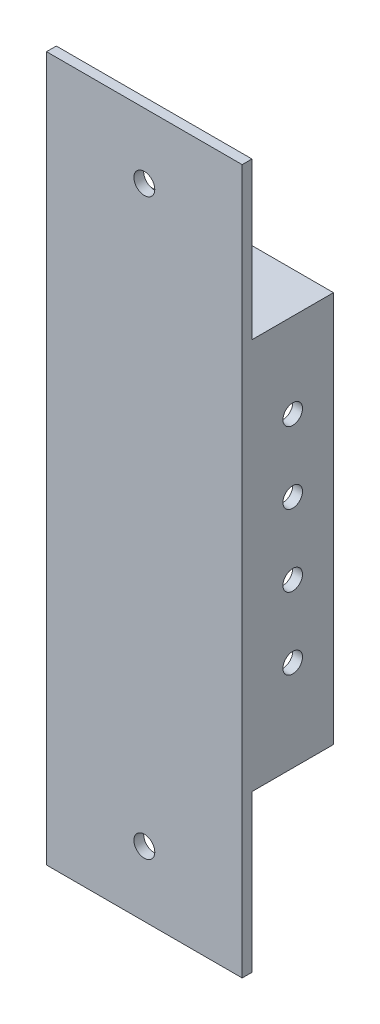
SolidWorks part; units mm, degrees
ref_plane "Front Plane" through (0, 0, 0) normal (0, 0, 1) x (1, 0, 0)
ref_plane "Top Plane" through (0, 0, 0) normal (0, 1, 0) x (1, 0, 0)
ref_plane "Right Plane" through (0, 0, 0) normal (1, 0, 0) x (0, 0, -1)
other "Configuration Table"
sketch "Sketch1" plane through (0, 0, 0) normal (0, 0, 1) x (1, 0, 0)
  line L1 (-300, -600) -> (300, -600)
  line L2 (-300, -600) -> (-300, 600)
  line L3 (-300, 600) -> (300, 600)
  line L4 (300, -600) -> (300, 600)
  line L5 (-300, -600) -> (300, 600) construction
  line L6 (-300, 600) -> (300, -600) construction
  point P0 (0, 0)
  dimension "D1" = 600
  dimension "D2" = 1200
extrude "Boss-Extrude1" add sketch "Sketch1" along normal blind 30
sketch "Sketch3" plane through (0, 0, 0) normal (0, 0, -1) x (-1, 0, 0)
  line L1 (-300, 600) -> (300, 600)
  line L2 (-300, 600) -> (-300, -600)
  line L3 (-300, -600) -> (300, -600)
  line L4 (300, 600) -> (300, -600)
  line L5 (-270, 570) -> (270, 570)
  line L6 (-270, 570) -> (-270, -570)
  line L7 (-270, -570) -> (270, -570)
  line L8 (270, 570) -> (270, -570)
  dimension "D1" = 30
  dimension "D2" = 30
  dimension "D3" = 30
  dimension "D4" = 30
extrude "Boss-Extrude2" add sketch "Sketch3" along normal blind 250
sketch "Sketch4" plane through (-300, 0, 0) normal (-1, 0, 0) x (0, 0, 1)
  line L0 (-125, 600) -> (-125, -600) construction
  line L1 (30, 600) -> (-250, 600) construction
  line L2 (30, -600) -> (-250, -600) construction
  line L3 (-250, -600) -> (-250, 600) construction
  circle A0 centre (-125, 340) radius 30
  dimension "D2" = 60
  dimension "D1" = 125
  dimension "D3" = 260
extrude "Cut-Extrude2" cut sketch "Sketch4" against normal blind 660
pattern_linear "LPattern1" count 4 spacing 220 along (0, -1, 0) of "Cut-Extrude2"
sketch "Sketch5" plane through (0, 0, -250) normal (0, 0, -1) x (-1, 0, 0)
  line L0 (-300, 600) -> (-300, -600) construction
  line L1 (300, 600) -> (-300, 600) construction
  circle A0 centre (-285, 585) radius 5
  dimension "D2" = 15
  dimension "D3" = 10
  dimension "D1" = 15
extrude "Cut-Extrude3" cut sketch "Sketch5" against normal blind 20
pattern_linear "LPattern2" count 4 spacing 190 along (-1, 0, 0) of "Cut-Extrude3"
pattern_linear "LPattern3" count 4 spacing 390 along (0, -1, 0) of "Cut-Extrude3"
pattern_linear "LPattern4" count 2 spacing 570 along (-1, 0, 0) of "LPattern3"
pattern_linear "LPattern5" count 2 spacing 1170 along (0, -1, 0) of "LPattern2"
sketch "Sketch6" plane through (0, -600, 0) normal (0, -1, 0) x (1, 0, 0)
  line L0 (300, 30) -> (300, -250) construction
  line L1 (-300, 30) -> (300, 30)
  line L2 (-300, 30) -> (-300, 0)
  line L3 (-300, 0) -> (300, 0)
  line L4 (300, 30) -> (300, 0)
  dimension "D1" = 30
extrude "Boss-Extrude3" add sketch "Sketch6" along normal blind 480
sketch "Sketch8" plane through (0, 600, 0) normal (0, 1, 0) x (1, 0, 0)
  line L0 (300, -30) -> (300, 250) construction
  line L1 (-300, -30) -> (300, -30)
  line L2 (-300, -30) -> (-300, 0)
  line L3 (-300, 0) -> (300, 0)
  line L4 (300, -30) -> (300, 0)
  dimension "D1" = 30
extrude "Boss-Extrude4" add sketch "Sketch8" along normal blind 480
sketch "Sketch9" plane through (0, 0, 30) normal (0, 0, 1) x (1, 0, 0)
  line L0 (0, 1080) -> (0, -1080) construction
  line L1 (-300, 1080) -> (300, 1080) construction
  line L2 (300, -1080) -> (-300, -1080) construction
  circle A0 centre (0, 880) radius 32
  circle A1 centre (0, -880) radius 32
  dimension "D1" = 64
  dimension "D3" = 64
  dimension "D2" = 200
  dimension "D4" = 200
extrude "Cut-Extrude4" cut sketch "Sketch9" against normal blind 480
